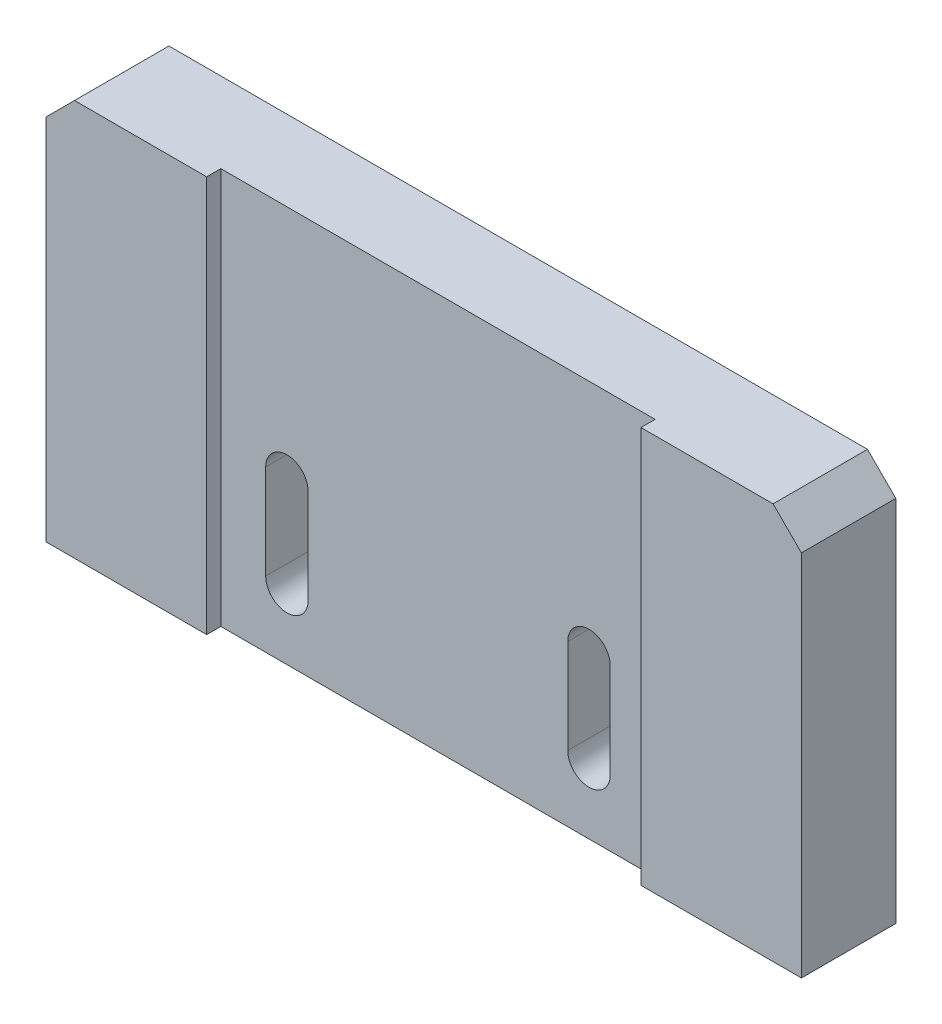
SolidWorks part; units mm, degrees
ref_plane "前视基准面" through (0, 0, 0) normal (0, 0, 1) x (1, 0, 0)
ref_plane "上视基准面" through (0, 0, 0) normal (0, 1, 0) x (1, 0, 0)
ref_plane "右视基准面" through (0, 0, 0) normal (1, 0, 0) x (0, 0, -1)
sketch "草图1" plane through (0, 0, 0) normal (0, 0, 1) x (1, 0, 0)
  line L1 (-40, -21) -> (40, -21)
  line L2 (-40, -21) -> (-40, 21)
  line L3 (-40, 21) -> (40, 21)
  line L4 (40, -21) -> (40, 21)
  line L5 (-40, -21) -> (40, 21) construction
  line L6 (-40, 21) -> (40, -21) construction
  point P0 (0, 0)
  dimension "D1" = 80
  dimension "D2" = 42
extrude "凸台-拉伸1" add sketch "草图1" along normal blind 10
sketch "草图2" plane through (0, 0, 10) normal (0, 0, 1) x (1, 0, 0)
  line L0 (40, 21) -> (-40, 21) construction
  line L1 (-23, -21) -> (23, -21)
  line L2 (-23, -21) -> (-23, 21)
  line L3 (-23, 21) -> (23, 21)
  line L4 (23, -21) -> (23, 21)
  line L5 (-23, -21) -> (23, 21) construction
  line L6 (-23, 21) -> (23, -21) construction
  point P0 (0, 0)
  dimension "D1" = 46
extrude "切除-拉伸1" cut sketch "草图2" against normal blind 1.5
chamfer "倒角1" distance 3 angle 45 2 edges at (-40, 21, 5) (40, 21, 5)
sketch "草图3" plane through (0, 0, 8.5) normal (0, 0, 1) x (1, 0, 0)
  line L0 (-16, -14) -> (-16, -4) construction
  line L1 (-18.25, -14) -> (-18.25, -4)
  line L2 (-13.75, -14) -> (-13.75, -4)
  line L3 (-23, -21) -> (23, -21) construction
  arc A0 (-18.25, -14) -> (-13.75, -14) centre (-16, -14) ccw
  arc A1 (-13.75, -4) -> (-18.25, -4) centre (-16, -4) ccw
  point P2 (-16, -9)
  dimension "D1" = 2.25
  dimension "D2" = 16
  dimension "D3" = 10
  dimension "D4" = 12
extrude "切除-拉伸2" cut sketch "草图3" against normal up to next
mirror "镜向1" about plane through (0, 0, 0) normal (1, 0, 0) of "切除-拉伸2"
